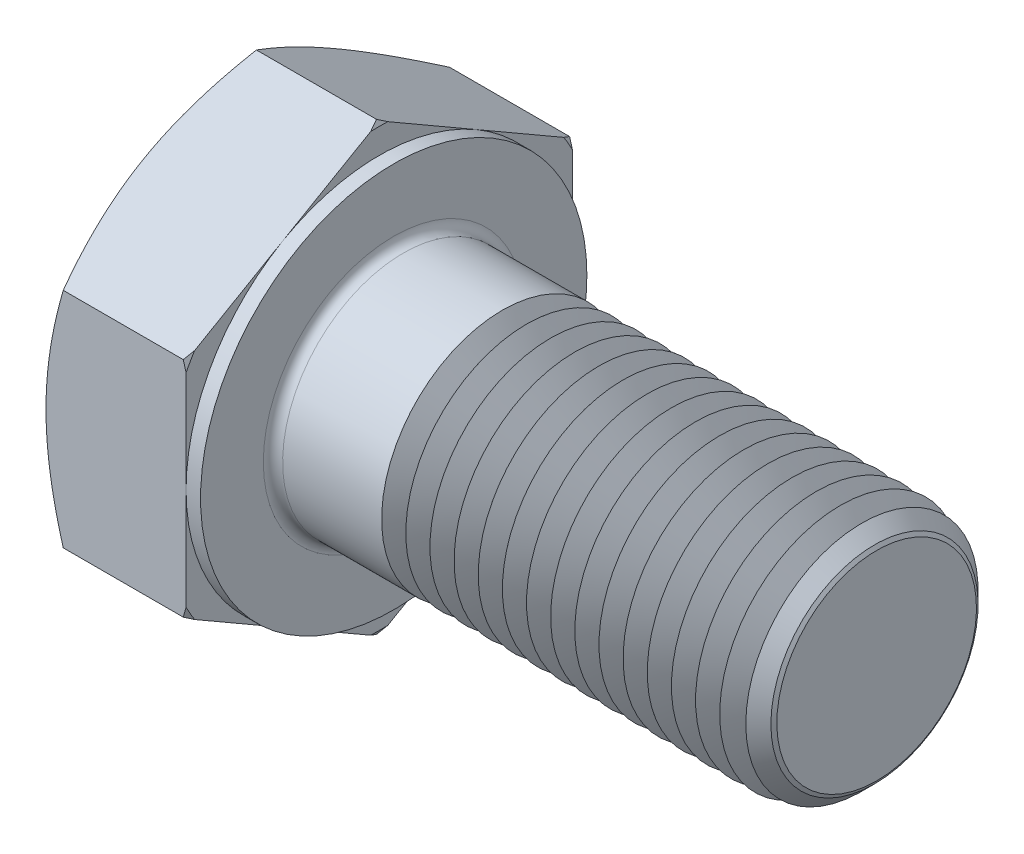
from build123d import *

# Parameters (mm, degrees)
EXTRUDE_393_DEPTH      = 6.4
SKETCH_4_W             = 0.6
SKETCH_4_H             = 11.237604307
CHAMFER_2072_SIZE      = 0.8
FILLET_2117_R          = 0.4
PATTERN_LINEAR_1_COUNT = 16
PATTERN_LINEAR_1_PITCH = 1


with BuildPart() as part:
    # 草图1 → Extrude 393 (new body)
    with BuildSketch(Plane(origin=(0, 0, 0), x_dir=(0, 0, -1), z_dir=(1, 0, 0))):
        Polygon((8, 4.618802154), (8, -4.618802154), (0, -9.237604307), (-8, -4.618802154), (-8, 4.618802154), (0, 9.237604307), align=None)
    extrude(amount=EXTRUDE_393_DEPTH)

    # 草图2 → 凸台-旋转1 (revolve)
    with BuildSketch(Plane.XY, mode=Mode.PRIVATE) as revolve_1_sk:
        Polygon((0, 0), (26.4, 0), (26.4, 4.134), (26.4, 5), (0, 5), align=None)
    revolve(revolve_1_sk.sketch.rotate(Axis((0, 0, 0), (1, 0, 0)), 90), axis=Axis((0, 0, 0), (1, 0, 0)))

    # 草图3 → 切除-旋转1 (revolve, cut)
    with BuildSketch(Plane.XY):
        Polygon((0, 8), (3.601282526, 14.237604307), (3.601282526, 19.237604307), (-10, 19.237604307), (-10, 8), align=None)
    revolve(axis=Axis((0, 0, 0), (1, 0, 0)), mode=Mode.SUBTRACT)

    # 草图5 → 切除-旋转2 (revolve, cut)
    with BuildSketch(Plane.XY):
        Polygon((6.4, 8), (2.798717474, 14.237604307), (2.798717474, 19.237604307), (12.798717474, 19.237604307), (12.798717474, 8), align=None)
    revolve(axis=Axis((0, 0, 0), (1, 0, 0)), mode=Mode.SUBTRACT)

    # 草图4 → 切除-旋转3 (revolve, cut)
    with BuildSketch(Plane.XY, mode=Mode.PRIVATE) as cut_revolve_3_sk:
        with Locations((6.1, 13.618802154)):
            Rectangle(SKETCH_4_W, SKETCH_4_H)
    revolve(cut_revolve_3_sk.sketch.rotate(Axis((0, 0, 0), (1, 0, 0)), 270), axis=Axis((0, 0, 0), (1, 0, 0)), mode=Mode.SUBTRACT)

    # Chamfer 2072
    chamfer_2072_edges = [part.edges().sort_by_distance(p)[0] for p in [
        (26.4, 0, -5),
    ]]
    chamfer(chamfer_2072_edges, length=CHAMFER_2072_SIZE)

    # Fillet 2117
    fillet_2117_edges = [part.edges().sort_by_distance(p)[0] for p in [
        (6.4, 0, -5),
    ]]
    fillet(fillet_2117_edges, radius=FILLET_2117_R)

    # 草图6 → 切除-旋转4 (revolve, cut)
    with BuildSketch(Plane.XY):
        Polygon((11.4, -4.134), (10.900014667, -5), (10.900014667, -6.25), (11.899985333, -6.25), (11.899985333, -5), align=None)
    cut_revolve_4 = revolve(axis=Axis((-3.175, 0, 0), (1, 0, 0)), mode=Mode.SUBTRACT)

    # 阵列(线性)1: 切除-旋转4 ×16
    with Locations(*[(i * PATTERN_LINEAR_1_PITCH, 0, 0) for i in range(1, PATTERN_LINEAR_1_COUNT)]):
        add(cut_revolve_4, mode=Mode.SUBTRACT)


solid = part.part
